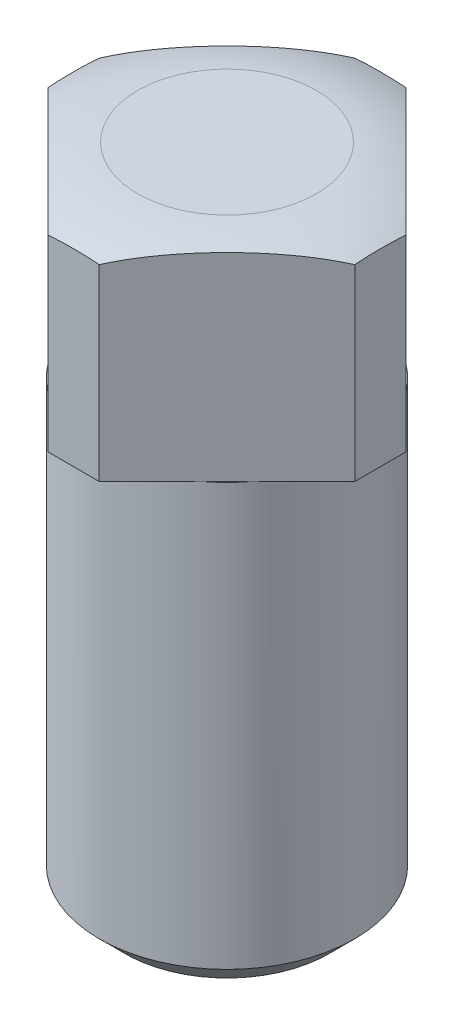
from build123d import *

# Parameters (mm, degrees)
CHAMFER1_SIZE       = 1
SKETCH2_R           = 11.978178672
CUT_EXTRUDE2_DEPTH  = 8
SKETCH4_R           = 5
BOSS_EXTRUDE1_DEPTH = 1.5
CHAMFER2_SIZE       = 1


with BuildPart() as part:
    # Sketch1 → Revolve1 (revolve)
    with BuildSketch(Plane.XY, mode=Mode.PRIVATE) as revolve1_sk:
        Polygon((0, 0), (0, 24), (10, 24), (10, 16), (5, 16), (5, 0), align=None)
    revolve(revolve1_sk.sketch.rotate(Axis((0, 0, 0), (0, 1, 0)), 90), axis=Axis((0, 0, 0), (0, 1, 0)))

    # Chamfer1
    chamfer1_edges = [part.edges().sort_by_distance(p)[0] for p in [
        (0, 0, 5),
    ]]
    chamfer(chamfer1_edges, length=CHAMFER1_SIZE)

    # Sketch2 → Cut-Extrude2 (cut)
    with BuildSketch(Plane(origin=(0, 24, 0), x_dir=(1, 0, 0), z_dir=(0, 1, 0))):
        Circle(SKETCH2_R)
        Polygon((-1, 6), (1, 6), (6, 1), (6, -1), (1, -6), (-1, -6), (-6, -1), (-6, 1), align=None, mode=Mode.SUBTRACT)
    extrude(amount=-CUT_EXTRUDE2_DEPTH, mode=Mode.SUBTRACT)

    # Sketch3 → Cut-Revolve1 (revolve, cut)
    with BuildSketch(Plane.XY, mode=Mode.PRIVATE) as cut_revolve1_sk:
        with BuildLine():
            Line((3.5, 24), (5.57579334, 25.302795294))
            Line((5.57579334, 25.302795294), (6.462708925, 23.688216178))
            Line((6.462708925, 23.688216178), (6.758347453, 22.996814774))
            ThreePointArc((6.758347453, 22.996814774), (5.187612361, 23.688216178), (3.5, 24))
        make_face()
    revolve(cut_revolve1_sk.sketch.rotate(Axis((0, 0, 0), (0, 1, 0)), 90), axis=Axis((0, 0, 0), (0, 1, 0)), mode=Mode.SUBTRACT)

    # Sketch4 → Boss-Extrude1 (add, symmetric)
    with BuildSketch(Plane.XZ):
        with Locations(Location((0, 0, 0), (0, 0, 270))):
            Circle(SKETCH4_R)
    extrude(amount=BOSS_EXTRUDE1_DEPTH, both=True)

    # Chamfer2
    chamfer2_edges = [part.edges().sort_by_distance(p)[0] for p in [
        (0, -1.5, 5),
    ]]
    chamfer(chamfer2_edges, length=CHAMFER2_SIZE)


solid = part.part
